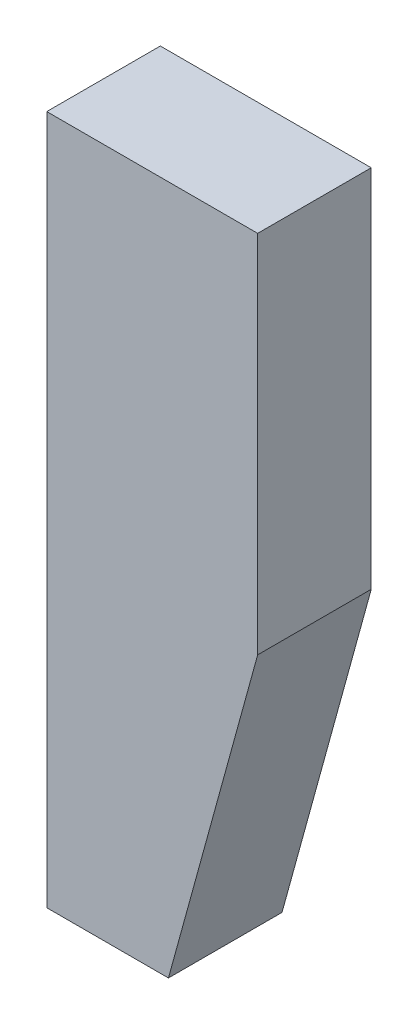
from build123d import *

# Parameters (mm, degrees)
EXTRUDE_1_DEPTH = 7


with BuildPart() as part:
    # 草图1 → 凸台-拉伸1 (new, symmetric)
    with BuildSketch(Plane.XY):
        Polygon((0, 0), (0, 85), (26, 85), (26, 40), (15, 0), align=None)
    extrude(amount=EXTRUDE_1_DEPTH, both=True)


solid = part.part
